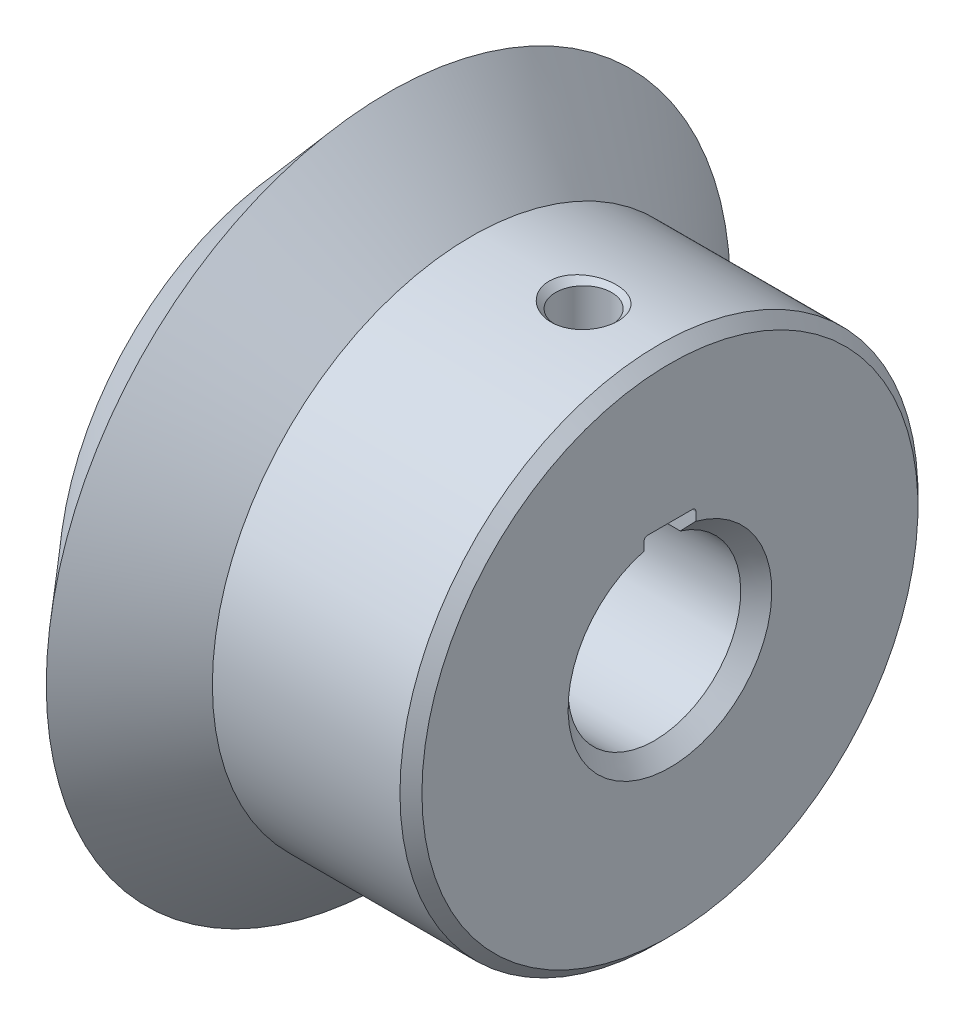
from build123d import *

# Parameters (mm, degrees)
CUT_EXTRUDE_1_DEPTH = 21.26


with BuildPart() as part:
    # 草图1 → 旋转1 (revolve)
    with BuildSketch(Plane.XY, mode=Mode.PRIVATE) as revolve_1_sk:
        Polygon((-21.26, 14.14569447), (-19, 11.85), (-19, 5), (0, 5), (0, 14.363603897), (-0.636396103, 15), (-11.5, 15), (-16.31, 19.81), align=None)
    revolve(revolve_1_sk.sketch.rotate(Axis((0, 0, 0), (-1, 0, 0)), 270), axis=Axis((0, 0, 0), (-1, 0, 0)))

    # 草图2 → 切除-旋转1 (revolve, cut)
    with BuildSketch(Plane.XY, mode=Mode.PRIVATE) as cut_revolve_1_sk:
        Polygon((-19, 0), (-19, 5.9), (-18.1, 5), (-0.9, 5), (0, 5.9), (0, 0), align=None)
    revolve(cut_revolve_1_sk.sketch.rotate(Axis((0, 0, 0), (-1, 0, 0)), 270), axis=Axis((0, 0, 0), (-1, 0, 0)), mode=Mode.SUBTRACT)

    # 草图3 → 切除-旋转2 (revolve, cut)
    with BuildSketch(Plane(origin=(-5, 0, 0), x_dir=(0, 0, -1), z_dir=(1, 0, 0)), mode=Mode.PRIVATE) as cut_revolve_2_sk:
        Polygon((0, 15), (2, 15), (1.621, 14.621), (1.621, 4.582575695), (0, 4.582575695), align=None)
    revolve(cut_revolve_2_sk.sketch.rotate(Axis((-5, 4.582575695, 0), (0, 1, 0)), 180), axis=Axis((-5, 4.582575695, 0), (0, 1, 0)), mode=Mode.SUBTRACT)

    # 草图4 → 切除-拉伸1 (cut)
    with BuildSketch(Plane(origin=(0, 0, 0), x_dir=(0, 0, -1), z_dir=(1, 0, 0))):
        with BuildLine():
            Line((-1.5, 0), (1.5, 0))
            Line((1.5, 0), (1.5, 6.2))
            ThreePointArc((1.5, 6.2), (1.441421356, 6.341421356), (1.3, 6.4))
            Line((1.3, 6.4), (-1.3, 6.4))
            ThreePointArc((-1.3, 6.4), (-1.441421356, 6.341421356), (-1.5, 6.2))
            Line((-1.5, 6.2), (-1.5, 0))
        make_face()
    extrude(amount=-CUT_EXTRUDE_1_DEPTH, mode=Mode.SUBTRACT)


solid = part.part
